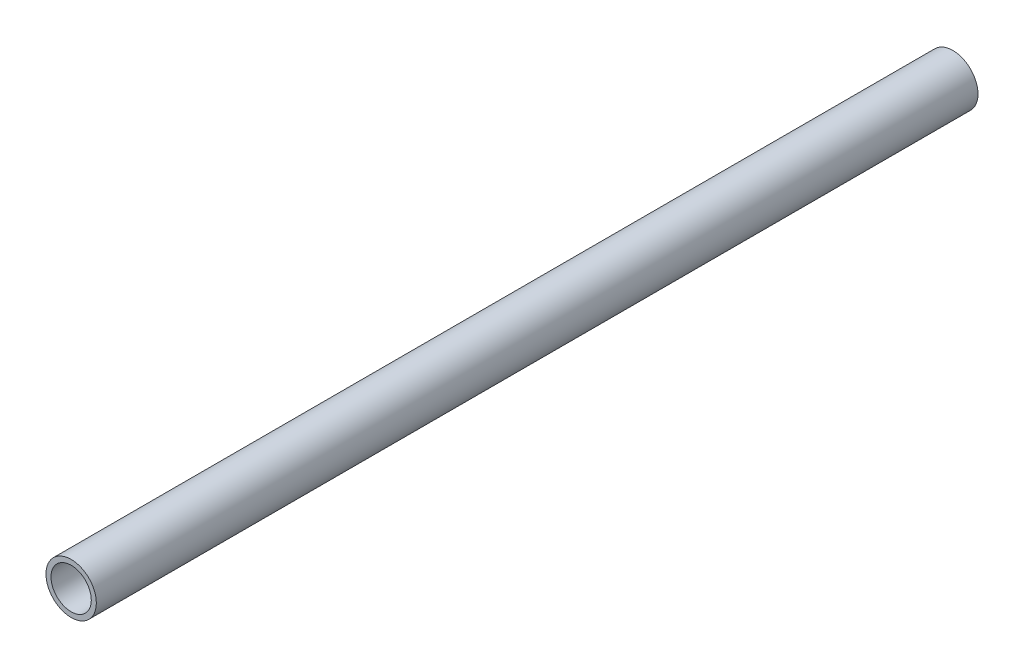
from build123d import *

# Parameters (mm, degrees)
SKETCH_1_R      = 10
SKETCH_1_R_2    = 8
EXTRUDE_1_DEPTH = 350


with BuildPart() as part:
    # 草图1 → 拉伸-薄壁1 (new body)
    with BuildSketch(Plane.XY):
        Circle(SKETCH_1_R)
        Circle(SKETCH_1_R_2, mode=Mode.SUBTRACT)
    extrude(amount=EXTRUDE_1_DEPTH)


solid = part.part
